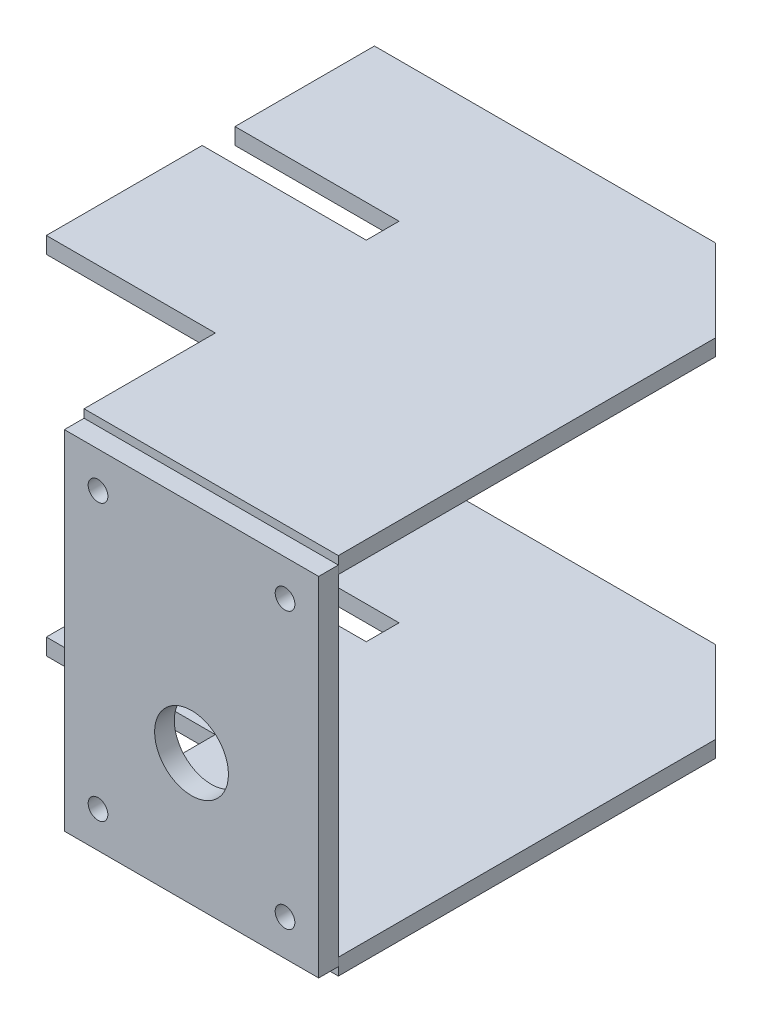
SolidWorks part; units mm, degrees
material "K"
ref_plane "Front" through (0, 0, 0) normal (0, 0, 1) x (1, 0, 0)
ref_plane "Top" through (0, 0, 0) normal (0, 1, 0) x (1, 0, 0)
ref_plane "Right" through (0, 0, 0) normal (1, 0, 0) x (0, 0, -1)
sketch "Sketch1" plane through (0, 0, 0) normal (0, 0, 1) x (1, 0, 0)
  line L1 (77.5, -106) -> (-77.5, -106)
  line L2 (77.5, -106) -> (77.5, 106)
  line L3 (77.5, 106) -> (-77.5, 106)
  line L4 (-77.5, -106) -> (-77.5, 106)
  line L5 (0, 106) -> (0, -106) construction
  line L6 (77.5, 0) -> (-77.5, 0) construction
  point P0 (0, 0)
  dimension "D1" = 155
  dimension "D2" = 212
extrude "Boss-Extrude1" add sketch "Sketch1" along normal blind 12
sketch "Sketch2" plane through (0, 0, 0) normal (0, 0, -1) x (-1, 0, 0)
  line L0 (0, 106) -> (0, -106) construction
  line L1 (-77.5, 106) -> (77.5, 106) construction
  line L2 (77.5, -106) -> (-77.5, -106) construction
sketch "Sketch3" plane through (0, 0, 0) normal (0, 0, -1) x (-1, 0, 0)
  line L1 (57, -84) -> (-57, -84) construction
  line L2 (57, -84) -> (57, 84) construction
  line L3 (57, 84) -> (-57, 84) construction
  line L4 (-57, -84) -> (-57, 84) construction
  line L5 (0, 84) -> (0, -84) construction
  line L6 (57, 0) -> (-57, 0) construction
  line L7 (0, 106) -> (0, -106) construction
  dimension "D1" = 168
  dimension "D2" = 114
hole_wizard "Ø12.0 (12) Diameter Hole1" positions "Sketch5" profile "Sketch4" hole size "Ø12.0" standard "GB"
sketch "Sketch5" plane through (0, 0, 0) normal (0, 0, -1) x (-1, 0, 0)
  point P0 (-57, 84)
  point P3 (57, 84)
  point P6 (-57, -84)
  point P9 (57, -84)
sketch "Sketch4" plane through (57, 84, 0) normal (1, 0, 0) x (0, 1, 0)
  line L0 (0, 0) -> (0, 12)
  line L1 (0, 12) -> (6, 12)
  line L2 (6, 12) -> (6, 0)
  line L5 (6, 0) -> (0, 0)
  line L11 (0, -6.35) -> (0, 107.95) construction
  dimension "通孔孔直径" = 12
  dimension "通孔孔深度" = 12
sketch "Sketch8" plane through (0, 106, 0) normal (0, 1, 0) x (1, 0, 0)
  line L3 (77.5, 0) -> (-77.5, 0)
  line L6 (0, 0) -> (0, 167.9322) construction
  line L7 (77.5, 0) -> (77.5, 280)
  line L8 (-180.5, 280) -> (-180.5, 80)
  line L9 (77.5, 280) -> (-180.5, 280)
  line L10 (-77.5, 80) -> (-180.5, 80)
  line L11 (-77.5, 0) -> (-77.5, 80)
  dimension "D1" = 80
  dimension "D2" = 200
  dimension "D3" = 258
extrude "Boss-Extrude2" add sketch "Sketch8" along normal mid plane 10 separate body
chamfer "Chamfer1" distance 50 angle 45
mirror "Mirror1" about plane through (0, 0, 0) normal (0, 1, 0)
sketch "Sketch9" plane through (0, 0, 0) normal (0, 0, -1) x (-1, 0, 0)
  circle A0 centre (0, -26) radius 22.5
  dimension "D1" = 45
extrude "Cut-Extrude2" cut sketch "Sketch9" against normal up to next
sketch "Sketch10" plane through (0, 111, 0) normal (0, 1, 0) x (1, 0, 0)
  line L0 (-180.5, 280) -> (-180.5, 80) construction
  line L1 (-180.5, 195) -> (-80.5, 195)
  line L2 (-180.5, 195) -> (-180.5, 175)
  line L3 (-180.5, 175) -> (-80.5, 175)
  line L4 (-80.5, 195) -> (-80.5, 175)
  line L5 (-180.5, 80) -> (-77.5, 80) construction
  dimension "D1" = 100
  dimension "D2" = 20
  dimension "D3" = 95
extrude "Cut-Extrude3" cut sketch "Sketch10" against normal through all
equation "\"零件重量\"= IIF ( \"SW-质量\" > 100 , int ( \"SW-质量\" ) , \"SW-质量\" )"
